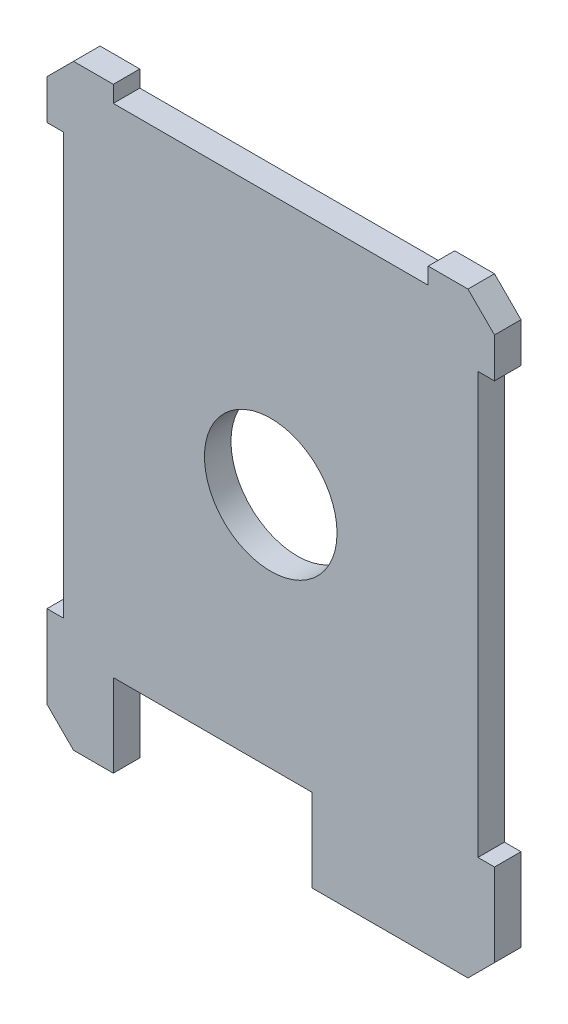
SolidWorks part; units mm, degrees
ref_plane "前视基准面" through (0, 0, 0) normal (0, 0, 1) x (1, 0, 0)
ref_plane "上视基准面" through (0, 0, 0) normal (0, 1, 0) x (1, 0, 0)
ref_plane "右视基准面" through (0, 0, 0) normal (1, 0, 0) x (0, 0, -1)
sketch "草图1" plane through (0, 0, 0) normal (0, 0, 1) x (1, 0, 0)
  line L1 (-67.5, -90) -> (67.5, -90)
  line L2 (-67.5, -90) -> (-67.5, 90)
  line L3 (-67.5, 90) -> (67.5, 90)
  line L4 (67.5, -90) -> (67.5, 90)
  line L5 (-67.5, -90) -> (67.5, 90) construction
  line L6 (-67.5, 90) -> (67.5, -90) construction
  point P0 (0, 0)
  dimension "D1" = 135
  dimension "D2" = 180
extrude "凸台-拉伸1" add sketch "草图1" along normal blind 8
sketch "草图2" plane through (0, 0, 8) normal (0, 0, 1) x (1, 0, 0)
  line L0 (67.5, 90) -> (-67.5, 90) construction
  line L1 (-47.5, 90) -> (47.5, 90)
  line L2 (-47.5, 90) -> (-47.5, 85)
  line L3 (-47.5, 85) -> (47.5, 85)
  line L4 (47.5, 90) -> (47.5, 85)
  line L5 (-67.5, 90) -> (-67.5, -90) construction
  line L6 (67.5, -90) -> (67.5, 90) construction
  line L7 (-47.5, -90) -> (-47.5, -65)
  line L8 (-67.5, -90) -> (67.5, -90) construction
  line L9 (-47.5, -65) -> (12.5, -65)
  line L10 (12.5, -65) -> (12.5, -90)
  line L11 (-67.5, 70) -> (-62.5, 70)
  line L12 (-62.5, 70) -> (-62.5, -57)
  line L13 (-62.5, -57) -> (-67.5, -57)
  line L14 (-67.5, -57) -> (-67.5, 70)
  line L15 (0, 0) -> (0, 68.4185) construction
  line L16 (67.5, -57) -> (67.5, 70)
  line L17 (62.5, -57) -> (67.5, -57)
  line L18 (62.5, 70) -> (62.5, -57)
  line L19 (67.5, 70) -> (62.5, 70)
  line L20 (-47.5, -90) -> (12.5, -90)
  dimension "D1" = 5
  dimension "D2" = 20
  dimension "D3" = 20
  dimension "D4" = 25
  dimension "D5" = 60
  dimension "D6" = 8
  dimension "D7" = 20
extrude "切除-拉伸1" cut sketch "草图2" against normal up to next
chamfer "倒角1" distance 8 angle 45 4 edges at (-67.5, 90, 4) (67.5, 90, 4) (67.5, -90, 4) (-67.5, -90, 4)
sketch "草图3" plane through (0, 0, 8) normal (0, 0, 1) x (1, 0, 0)
  line L0 (-62.5, 6.5) -> (62.5, 6.5) construction
  line L1 (-62.5, -57) -> (-62.5, 70) construction
  line L2 (62.5, 70) -> (62.5, -57) construction
  circle A0 centre (0, 6.5) radius 20
  dimension "D1" = 40
extrude "切除-拉伸2" cut sketch "草图3" against normal up to next
